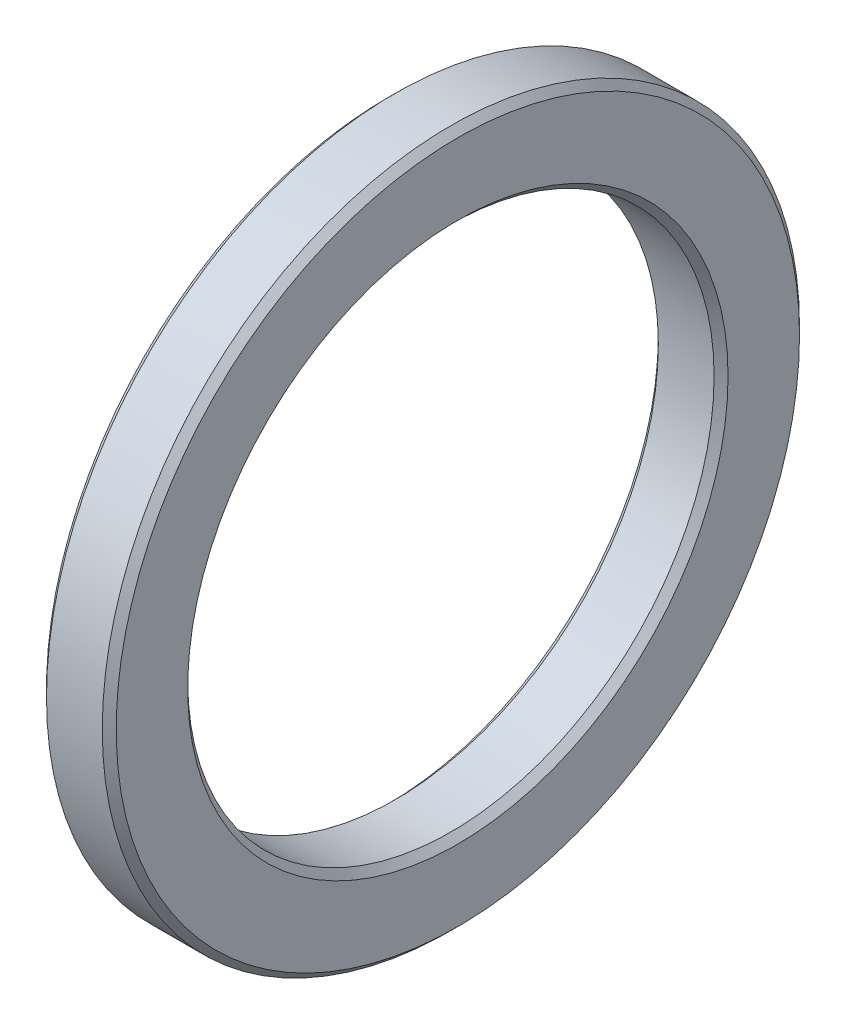
SolidWorks part; units mm, degrees
material "SUS201 T=2.0mm"
ref_plane "Front" through (0, 0, 0) normal (0, 0, 1) x (1, 0, 0)
ref_plane "Top" through (0, 0, 0) normal (0, 1, 0) x (1, 0, 0)
ref_plane "Right" through (0, 0, 0) normal (1, 0, 0) x (0, 0, -1)
sketch "草图1" plane through (0, 0, 0) normal (1, 0, 0) x (0, 0, -1)
  circle A0 centre (0, 0) radius 10
  circle A1 centre (0, 0) radius 7.55
  dimension "D1" = 15.1
  dimension "D2" = 20
extrude "凸台-拉伸1" add sketch "草图1" along normal blind 2
chamfer "倒角1" distance 0.2 angle 45 4 edges at (2, 0, -7.55) (2, 0, -10) (0, 0, -7.55) (0, 0, -10)
